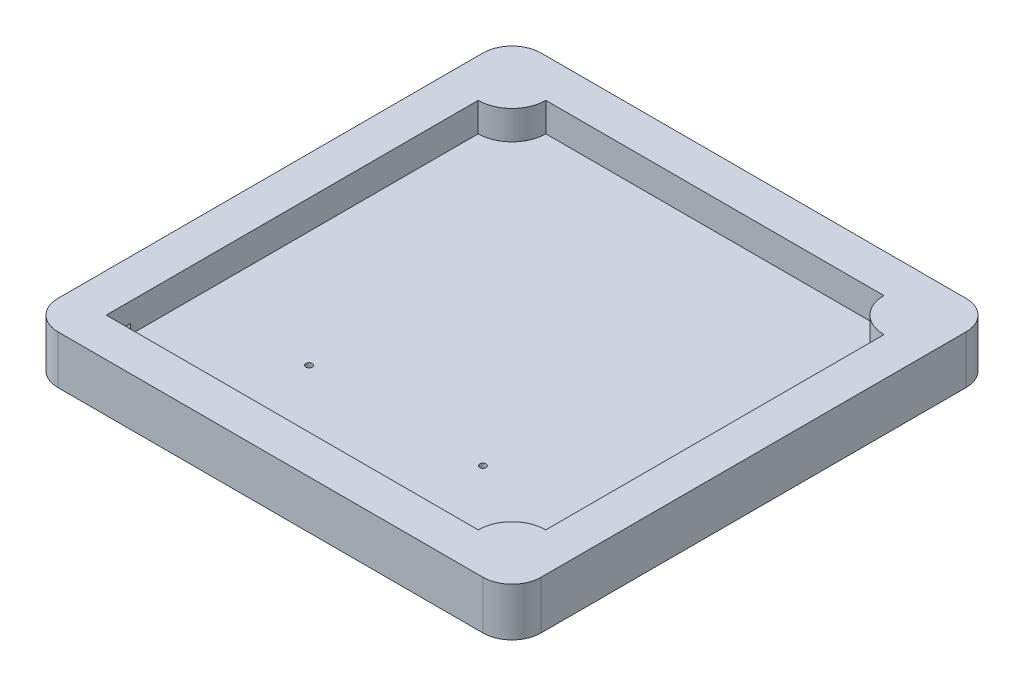
from build123d import *

# Parameters (mm, degrees)
BOSS_EXTRUDE1_DEPTH                                  = 50
CUT_EXTRUDE1_DEPTH                                   = 30
SKETCH3_R                                            = 25
CUT_EXTRUDE2_DEPTH                                   = 30
CBORE_FOR_M6_HEXAGON_HEAD_BOLTS_FULL_THR_D           = 6.6
CBORE_FOR_M6_HEXAGON_HEAD_BOLTS_FULL_THR_CBORE_D     = 13
CBORE_FOR_M6_HEXAGON_HEAD_BOLTS_FULL_THR_CBORE_DEPTH = 0.5
CUT_EXTRUDE8_DEPTH                                   = 30


with BuildPart() as part:
    # Sketch1 → Boss-Extrude1 (new body)
    with BuildSketch(Plane(origin=(0, 0, 0), x_dir=(1, 0, 0), z_dir=(0, 1, 0))):
        with BuildLine():
            Line((-220, -250), (220, -250))
            ThreePointArc((220, -250), (241.213203436, -241.213203436), (250, -220))
            Line((250, -220), (250, 220))
            ThreePointArc((250, 220), (241.213203436, 241.213203436), (220, 250))
            Line((220, 250), (-220, 250))
            ThreePointArc((-220, 250), (-241.213203436, 241.213203436), (-250, 220))
            Line((-250, 220), (-250, -220))
            ThreePointArc((-250, -220), (-241.213203436, -241.213203436), (-220, -250))
        make_face()
    extrude(amount=BOSS_EXTRUDE1_DEPTH)

    # Sketch2 → Cut-Extrude1 (cut)
    with BuildSketch(Plane(origin=(0, 50, 0), x_dir=(1, 0, 0), z_dir=(0, 1, 0))):
        with BuildLine():
            Line((-175, -210), (175, -210))
            ThreePointArc((175, -210), (185.251262658, -185.251262658), (210, -175))
            Line((210, -175), (210, 175))
            ThreePointArc((210, 175), (185.251262658, 185.251262658), (175, 210))
            Line((175, 210), (-175, 210))
            ThreePointArc((-175, 210), (-185.251262658, 185.251262658), (-210, 175))
            Line((-210, 175), (-210, -175))
            ThreePointArc((-210, -175), (-185.251262658, -185.251262658), (-175, -210))
        make_face()
    extrude(amount=-CUT_EXTRUDE1_DEPTH, mode=Mode.SUBTRACT)

    # Sketch3 → Cut-Extrude2 (cut)
    with BuildSketch(Plane.XZ):
        with Locations(Location((-210, 210, 0), (0, 0, 270))):
            Circle(SKETCH3_R)
        with Locations(Location((210, 210, 0), (0, 0, 90))):
            Circle(SKETCH3_R)
        with Locations(Location((210, -210, 0), (0, 0, 270))):
            Circle(SKETCH3_R)
        with Locations(Location((-210, -210, 0), (0, 0, 90))):
            Circle(SKETCH3_R)
    extrude(amount=-CUT_EXTRUDE2_DEPTH, mode=Mode.SUBTRACT)

    # CBORE for M6 Hexagon head bolts-Full thread-grade C1 (through all)
    with Locations(Plane.XZ):
        with Locations((90, 200), (-90, 200), (90, 120), (-90, 120)):
            CounterBoreHole(CBORE_FOR_M6_HEXAGON_HEAD_BOLTS_FULL_THR_D / 2, CBORE_FOR_M6_HEXAGON_HEAD_BOLTS_FULL_THR_CBORE_D / 2, CBORE_FOR_M6_HEXAGON_HEAD_BOLTS_FULL_THR_CBORE_DEPTH)

    # Sketch10 → Cut-Extrude8 (cut)
    with BuildSketch(Plane(origin=(0, 50, 0), x_dir=(1, 0, 0), z_dir=(0, 1, 0))):
        with BuildLine():
            Line((-210, -175), (-210, -210))
            Line((-210, -210), (-175, -210))
            ThreePointArc((-175, -210), (-185.251262658, -185.251262658), (-210, -175))
        make_face()
    extrude(amount=-CUT_EXTRUDE8_DEPTH, mode=Mode.SUBTRACT)


solid = part.part
